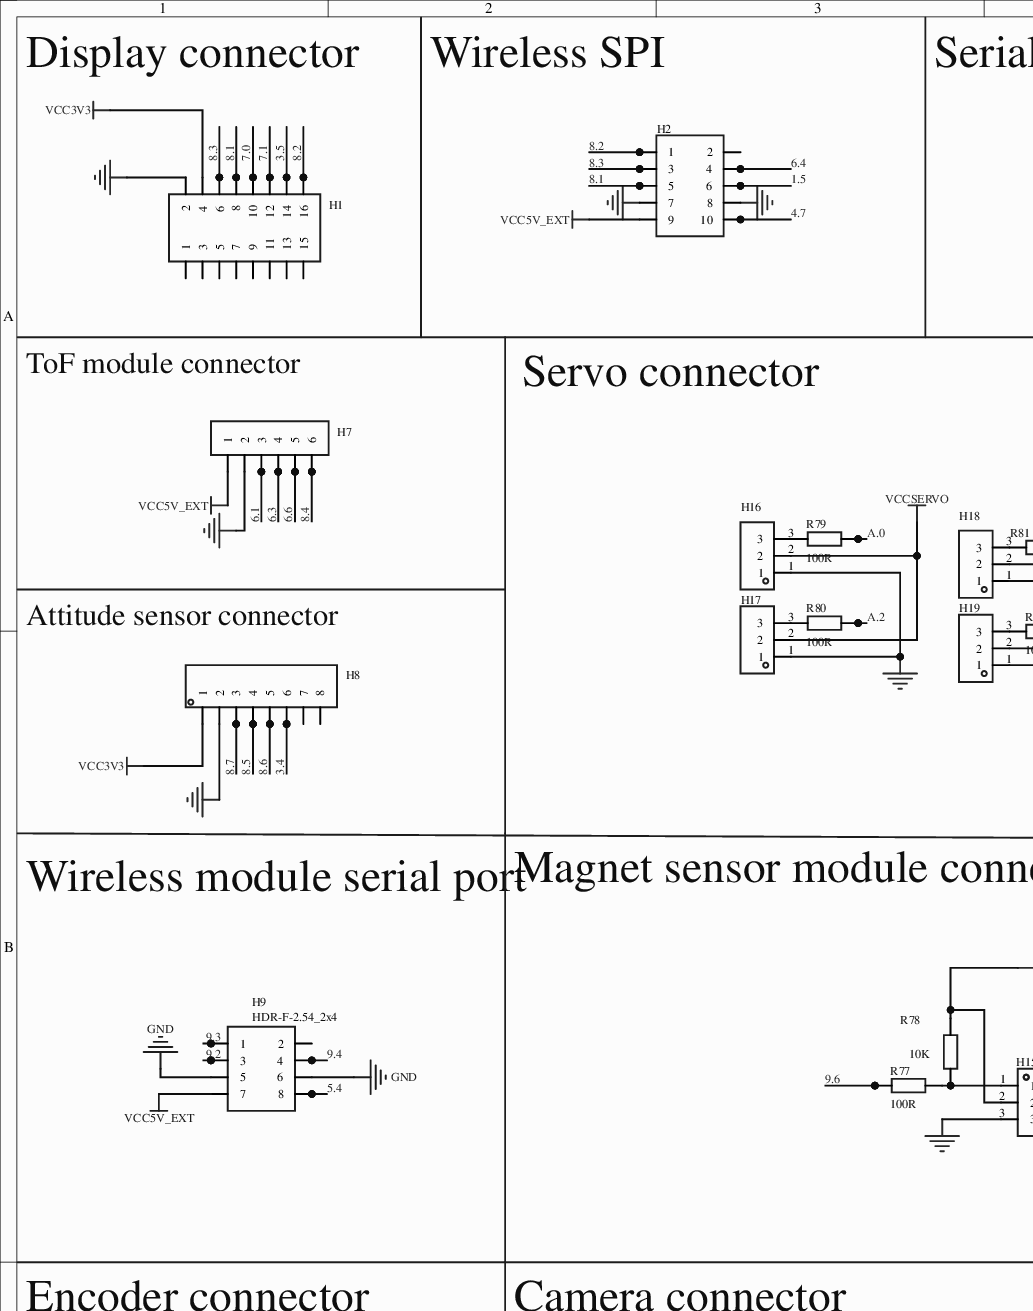
[diagram p0: MISC49918-4.schdoc, top left]
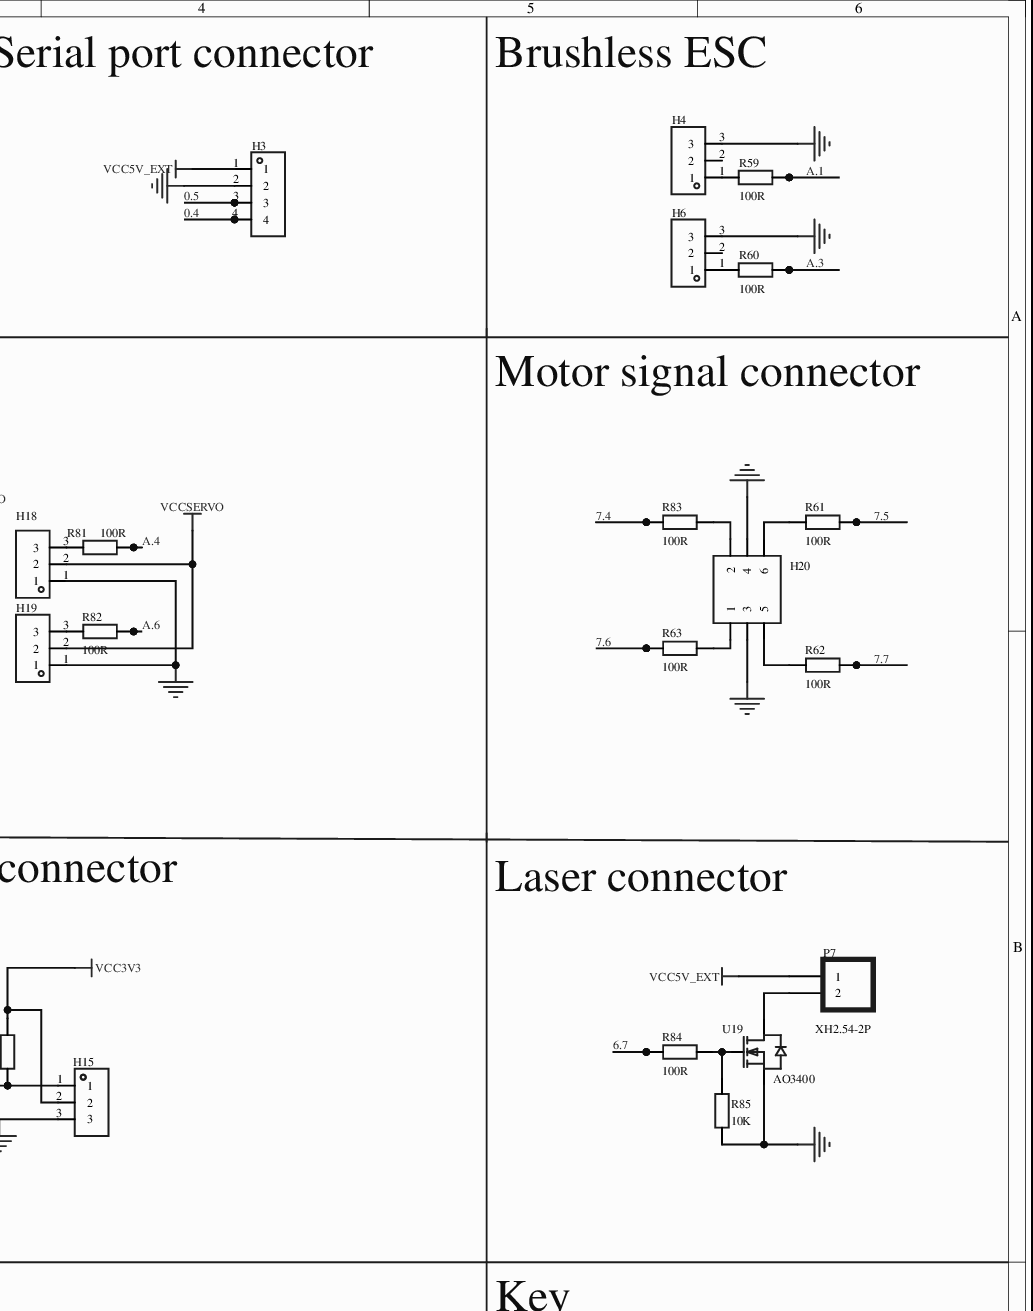
[diagram p1: MISC49918-4.schdoc, top right]
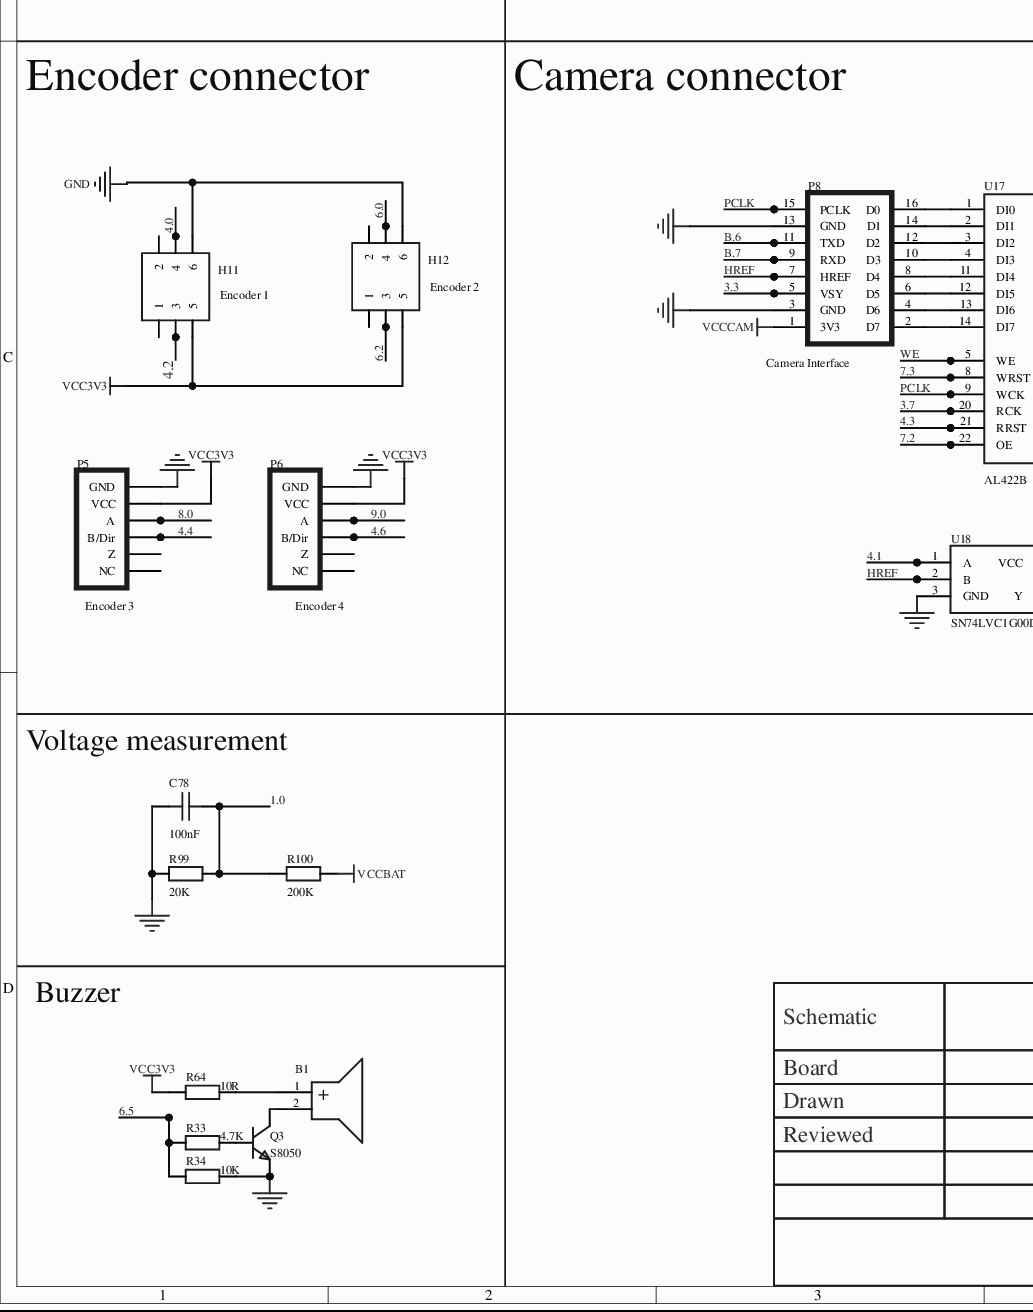
[diagram p2: MISC49918-4.schdoc, bottom left]
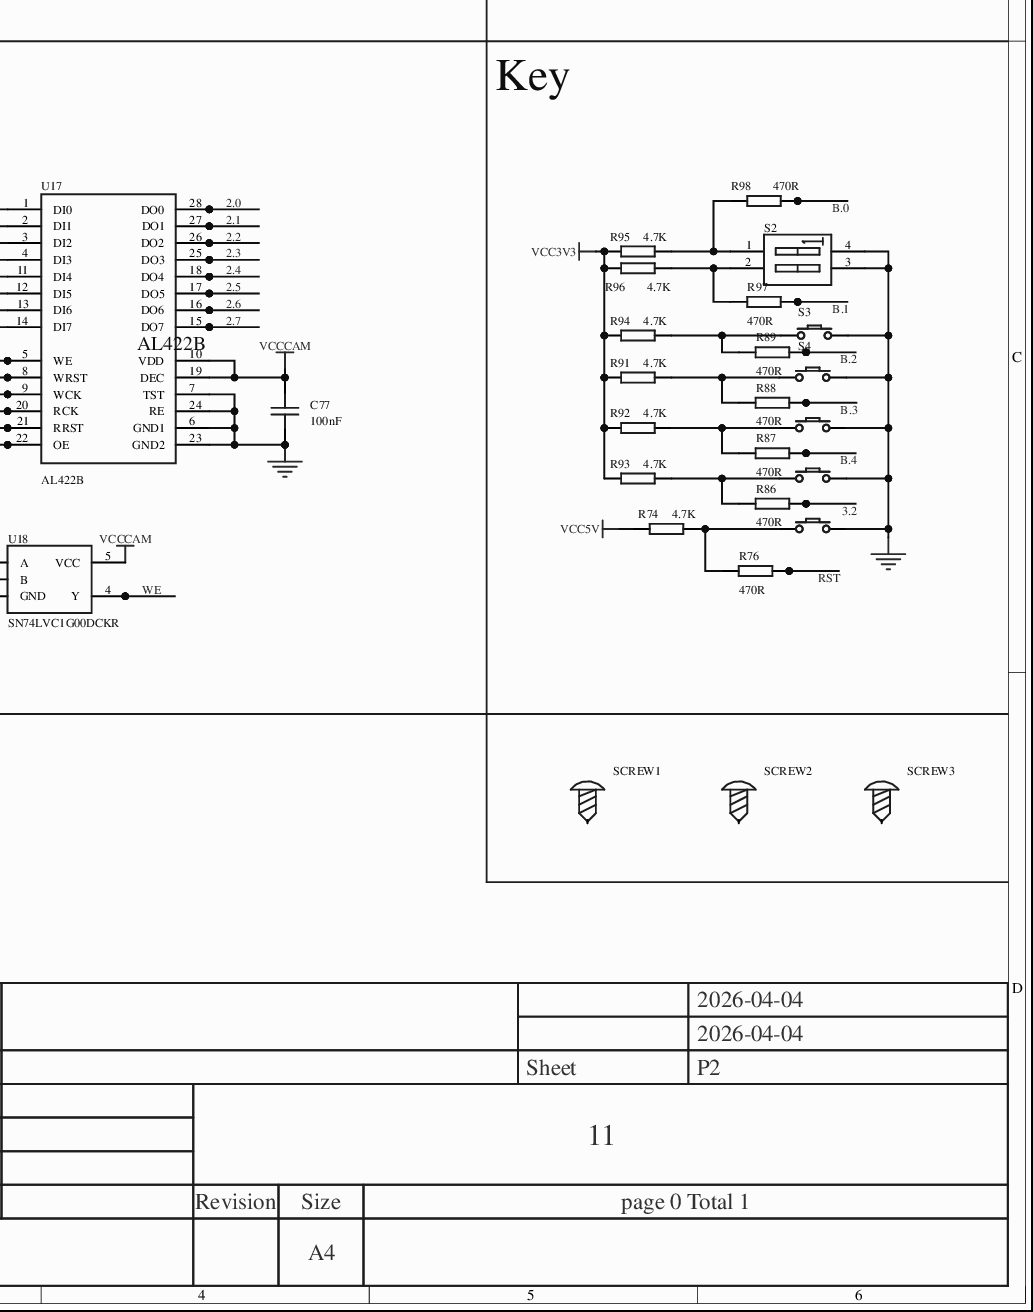
[diagram p3: MISC49918-4.schdoc, bottom right]
# Altium project MISC49918-2.PrjPcb (part 2 of 2)

## Sheet MISC49918-4.schdoc
size 297 x 381 mm; Version: V1.0; @Project Name: MISC49918; @Update Date: 2026-04-09; @Create Date: 2026-04-09; @Board Name: MISC49918; @Create Time: 13:05:40; @Page Count: 1; @Page No: 0; @Schematic Name: MISC49918; @Update Time: 13:05:40; Size: A4

### Parts
B1  3kHz  [BUZ-TH_BD9.0-P5.00-D0.6-FD]  (value not drawn)
C77  100nF  [C0603]
C78  100nF  [C0603]
H1  (no value)  [HDR-TH_16P-P2.54-V-F-R2-C8-S2.54-1]
H2  (no value)  [HDR-TH_10P-P2.54-V-F-R2-C5-S2.54]
H3  (no value)  [HDR-TH_4P-P2.54-V-M]
H4  (no value)  [HDR-TH_3P-P2.54-V-M]
H6  (no value)  [HDR-TH_3P-P2.54-V-M]
H7  (no value)  [HDR-TH_6P-P2.54-V-M-1]
H8  (no value)  [HDR-TH_8P-P2.54-V-M]
H9  HDR-F-2.54_2x4  [HDR-F-2.54_2X4]
H11  (no value)  [HDR-TH_6P-P2.54-V-R2-C3-S2.54_A2541WV-2X3P]
H12  (no value)  [HDR-TH_6P-P2.54-V-R2-C3-S2.54_A2541WV-2X3P]
H15  (no value)  [HDR-TH_3P-P2.54-V-M]
H16  (no value)  [HDR-TH_3P-P2.54-V-M]
H17  (no value)  [HDR-TH_3P-P2.54-V-M]
H18  (no value)  [HDR-TH_3P-P2.54-V-M]
H19  (no value)  [HDR-TH_3P-P2.54-V-M]
H20  (no value)  [HDR-TH_6P-P2.54-V-R2-C3-S2.54_A2541WV-2X3P]
P5  GH1.25-6P-SH new encoder board end, horizontal  [ECD-GH1.25-6P-SV]  (value not drawn)
P6  GH1.25-6P-SH new encoder board end, horizontal  [ECD-GH1.25-6P-SV]  (value not drawn)
P7  XH2.54-2P  [XH2.54-2P-DV]
P8  Camera Interface  [HDR2X8-F-High]
Q3  S8050  [SOT-23-3_L3.0-W1.7-P0.95-LS2.9-BR]
R33  4.7K  [R0603]
R34  10K  [R0603]
R59  100R  [R0603]
R60  100R  [R0603]
R61  100R  [R0603]
R62  100R  [R0603]
R63  100R  [R0603]
R64  10R  [R0603]
R74  4.7K  [RESC1608[0603]S-N]
R76  470R  [RESC1608[0603]S-N]
R77  100R  [R0603]
R78  10K  [R0603]
R79  100R  [R0603]
R80  100R  [R0603]
R81  100R  [R0603]
R82  100R  [R0603]
R83  100R  [R0603]
R84  100R  [R0603]
R85  10K  [R0603]
R86  470R  [RESC1608[0603]S-N]
R87  470R  [RESC1608[0603]S-N]
R88  470R  [RESC1608[0603]S-N]
R89  470R  [RESC1608[0603]S-N]
R91  4.7K  [RESC1608[0603]S-N]
R92  4.7K  [RESC1608[0603]S-N]
R93  4.7K  [RESC1608[0603]S-N]
R94  4.7K  [RESC1608[0603]S-N]
R95  4.7K  [RESC1608[0603]S-N]
R96  4.7K  [RESC1608[0603]S-N]
R97  470R  [RESC1608[0603]S-N]
R98  470R  [RESC1608[0603]S-N]
R99  20K  [R0603]
R100  200K  [R0603]
S2  SW DIP-2  [Code SW-2-DIP-2.54]  (value not drawn)
S3  KEY-TS1145  [TS-1199A]  (value not drawn)
S4  KEY-TS1145  [TS-1199A]  (value not drawn)
S5  KEY-TS1145  [TS-1199A]  (value not drawn)
S6  KEY-TS1145  [TS-1199A]  (value not drawn)
S7  KEY-TS1145  [TS-1199A]  (value not drawn)
SCREW1  (no value)  [M3螺丝]
SCREW2  (no value)  [M3螺丝]
SCREW3  (no value)  [M3螺丝]
U17  AL422B  [SOP-28]
U18  SN74LVC1G00DCKR  [SOT-353]
U19  AO3400  [SOT-23-3_L2.9-W1.3-P1.90-LS2.4-BL-2]

### Nets
GND: C77.1 C78.1 H1.2 H2.7 H2.8 H3.2 H4.3 H6.3 H7.2 H8.2 H9.5 H9.6 H11.6 H12.6 H15.3 H16.1 H17.1 H18.1 H19.1 H20.3 H20.4 P5.1(GND) P6.1(GND) P8.3(GND) P8.13(GND) Q3.2(E) R34.2 R85.1 R99.1 S2.3(B2) S2.4(B1) S3.1 S4.1 S5.1 S6.1 S7.1 U17.6(GND1) U17.7(TST) U17.23(GND2) U17.24(RE) U18.3(GND) U19.2(S)
VCC3V3: H1.4 H8.1 H11.5 H12.5 H15.2 P5.2(VCC) P6.2(VCC) R64.1 R78.2 R91.1 R92.1 R93.1 R94.1 R95.1 R96.1
VCC5V: R74.1
VCC5V_EXT: H2.9 H3.1 H7.1 H9.7 P7.1
VCCBAT: R100.2
VCCCAM: C77.2 P8.1(3V3) U17.10(VDD) U17.19(DEC) U18.5(VCC)
VCCSERVO: H16.2 H17.2 H18.2 H19.2
0.4: H3.4
0.5: H3.3
1.0: C78.2 R99.2 R100.1
1.5: H2.6
2.0: U17.28(DO0)
2.1: U17.27(DO1)
2.2: U17.26(DO2)
2.3: U17.25(DO3)
2.4: U17.18(DO4)
2.5: U17.17(DO5)
2.6: U17.16(DO6)
2.7: U17.15(DO7)
3.2: R86.1
3.3: P8.5(VSY)
3.4: H8.6
3.5: H1.14
3.7: U17.20(RCK)
4.0: H11.4
4.1: U18.1(A)
4.2: H11.3
4.3: U17.21(RRST)
4.4: P5.4(B/Dir)
4.6: P6.4(B/Dir)
4.7: H2.10
5.4: H9.8
6.0: H12.4
6.1: H7.3
6.2: H12.3
6.3: H7.4
6.4: H2.4
6.5: R33.1 R34.1
6.6: H7.5
6.7: R84.1
7.0: H1.10
7.1: H1.12
7.2: U17.22(OE)
7.3: U17.8(WRST)
7.4: R83.1
7.5: R61.2
7.6: R63.1
7.7: R62.2
8.0: P5.3(A)
8.1: H1.8 H2.5
8.2: H1.16 H2.1
8.3: H1.6 H2.3
8.4: H7.6
8.5: H8.4
8.6: H8.5
8.7: H8.3
9.0: P6.3(A)
9.2: H9.3
9.3: H9.1
9.4: H9.4
9.6: R77.1
A.0: R79.2
A.1: R59.2
A.2: R80.2
A.3: R60.2
A.4: R81.2
A.6: R82.2
B.0: R98.1
B.1: R97.1
B.2: R89.1
B.3: R88.1
B.4: R87.1
B.6: P8.11(TXD)
B.7: P8.9(RXD)
HREF: P8.7(HREF) U18.2(B)
PCLK: P8.15(PCLK) U17.9(WCK)
RST: R76.1
WE: U17.5(WE) U18.4(Y)
NetB1_1: B1.1(+) R64.2
NetB1_2: B1.2(-) Q3.3(C)
NetH4_1: H4.1 R59.1
NetH6_1: H6.1 R60.1
NetH15_1: H15.1 R77.2 R78.1
NetH16_3: H16.3 R79.1
NetH17_3: H17.3 R80.1
NetH18_3: H18.3 R81.1
NetH19_3: H19.3 R82.1
NetH20_1: H20.1 R63.2
NetH20_2: H20.2 R83.2
NetH20_5: H20.5 R62.1
NetH20_6: H20.6 R61.1
NetP7_2: P7.2 U19.3(D)
NetP8_2: P8.2(D7) U17.14(DI7)
NetP8_4: P8.4(D6) U17.13(DI6)
NetP8_6: P8.6(D5) U17.12(DI5)
NetP8_8: P8.8(D4) U17.11(DI4)
NetP8_10: P8.10(D3) U17.4(DI3)
NetP8_12: P8.12(D2) U17.3(DI2)
NetP8_14: P8.14(D1) U17.2(DI1)
NetP8_16: P8.16(D0) U17.1(DI0)
NetQ3_1: Q3.1(B) R33.2
NetR74_2: R74.2 R76.2 S7.2
NetR84_2: R84.2 R85.2 U19.1(G)
NetR86_2: R86.2 R93.2 S6.2
NetR87_2: R87.2 R92.2 S5.2
NetR88_2: R88.2 R91.2 S4.2
NetR89_2: R89.2 R94.2 S3.2
NetR95_2: R95.2 R98.2 S2.1(A1)
NetR96_2: R96.2 R97.2 S2.2(A2)

Not connected (* = marked no-connect by the designer): H1 1* 3* 5* 7* 9* 11* 13* 15*; H2 2*; H4 2*; H6 2*; H8 7* 8*; H9 2*; H11 1* 2*; H12 1* 2*; P5 5(Z)* 6(NC)*; P6 5(Z)* 6(NC)*; SCREW1 1*; SCREW2 1*; SCREW3 1*

### Notes on the sheet
- Display connector
- Wireless SPI
- Serial port connector
- Brushless ESC
- ToF module connector
- Servo connector
- Motor signal connector
- Attitude sensor connector
- Wireless module serial port
- Magnet sensor module connector
- Laser connector
- Encoder connector
- Camera connector
- Key
- (near H11) Encoder 1
- (near H12) Encoder 2
- (near P5) Encoder 3
- (near P6) Encoder 4
- (near C78) Voltage measurement
- Buzzer
- 2026-04-04
- Schematic
- Board
- Sheet
- P2
- Drawn
- Reviewed
- 11
- Revision
- Size
- A4
- page 0 Total 1

### Library data of the parts
B1 = HNB09A03: Drive method: active (built-in driver circuit); Construction: electromagnetic; Frequency: 3kHz; Sound pressure (SPL): 85dB@10cm;; Manufacturer: 华能; 3D Model: 13273335caac486e928bafb4d9fdf12d; 3D Model Transform: 354.33,354.33,0,90,0,0,-0.005,0,-177.165; Operating Voltage: 1.5V~4.5V; Current Consumption: 30mA; AddInBom: yes; ModelName: BUZ-TH_D9.0-H5.5-P5.0; Device: HNB09A03; Symbol: HNB09A03; LCSC Part Name: 电磁式有源一体蜂鸣器HNB09A03; Supplier Footprint: 插件,D=9mm; Datasheet: https://atta.szlcsc.com/upload/public/pdf/source/20170522/1495448326172.pdf; Oscillator Circuit: Active (built-in driver circuit); Technology Type: Electromagnetic; Sound Pressure Level (SPL): 85dB@10cm; Diameter (φD): 9mm; Length: -; Width: -; Height: 5.5mm; Operating Temperature: -20℃~+70℃; Supplier: LCSC; Supplier Part: C96102; Manufacturer Part: HNB09A03; Value: 3kHz; FootprintName: BUZ-TH_BD9.0-P5.00-D0.6-FD; ConvertToPcb: yes
C77 C78 = CAP_0603: Symbol: Capacitance; 3D Model: ac125912035d415993ca9572d50418b1; 3D Model Transform: 62.992,31.496,0,0,0,0,0,0,0; ConvertToPcb: yes; ModelName: C0603_L1.6-W0.8-H0.8; Device: CAP_0603; Supplier Footprint: 0603; Value: 100nF; FootprintName: C0603; AddInBom: yes
H1 = HDR-F_2.54_2x8: Symbol: HDR-F-2.54_2x8; 3D Model: f6b5f7d40ec74b809fbaeebc5002f6e0; 3D Model Transform: 799.99844,200,0,0,0,0,0,0,-118.11; ConvertToPcb: yes; ModelName: HDR2.54-F-LI-2X8P; Device: HDR-F_2.54_2x8; Supplier Part: C30734; Supplier Footprint: 插件; FootprintName: HDR-TH_16P-P2.54-V-F-R2-C8-S2.54-1; AddInBom: yes
H2 = HDR-F_2.54_2x5: Symbol: HDR-F-2.54_2x5; 3D Model: 86e5d65f54dd476391caab3fdb916824; 3D Model Transform: 499.999,200,0,0,0,0,0,0,-118.11; ConvertToPcb: yes; ModelName: HDR2.54-F-LI-2X5P; Device: HDR-F_2.54_2x5; Supplier Part: C92270; Supplier Footprint: 插件; FootprintName: HDR-TH_10P-P2.54-V-F-R2-C5-S2.54; AddInBom: yes
H3 = HDR-M_2.54_1x4P: Symbol: PZ254V-11-04P; 3D Model: 112f4d05e8d64e99ab9a333894bea4f9; 3D Model Transform: 399.999,104.7242,0,0,0,0,0,0,-118.11; ConvertToPcb: yes; ModelName: HDR-TH_4P-P2.54-M-LI-1X4P; Device: HDR-M_2.54_1x4P; Supplier Part: C492403; Supplier Footprint: 插件; FootprintName: HDR-TH_4P-P2.54-V-M; AddInBom: yes
H4 H6 H15-H19 = HDR-M_2.54_1x3P: 3D Model: bb473b6d38ff42a99216a4fcdbdcc4cb; 3D Model Transform: 299.9993964861481,99.99979882871602,454.3297999999999,0,0,0,0,0,-118.11024; AddInBom: yes; ModelName: HDR-TH_3P-P2.54-M-LI-1X3P; Device: HDR-M_2.54_1x3P; Symbol: HDR-M_2.54_1x3P; Supplier Part: C2937625; Supplier Footprint: 插件; FootprintName: HDR-TH_3P-P2.54-V-M; ConvertToPcb: yes
H7 = HDR-M_2.54_1x6P: Symbol: Header-Male-2.54_1x6; 3D Model: 60739dffc9b04830a286435b0fefbd4a; 3D Model Transform: 599.999,100,0,0,0,0,0,0,-118.11; ConvertToPcb: yes; ModelName: HDR2.54-M-LI-1X6P; Device: HDR-M_2.54_1x6P; Supplier Part: C37208; Supplier Footprint: 插件; FootprintName: HDR-TH_6P-P2.54-V-M-1; AddInBom: yes
H8 = HDR-M_2.54_1x8P: Symbol: Header-Male-2.54_1x8; 3D Model: f5b96e27511e49e38545e53df2320202; 3D Model Transform: 807.87244,98.425,0,0,0,0,0,0,-118.11; ConvertToPcb: yes; Device: HDR-M_2.54_1x8P; Supplier Part: C124381; Supplier Footprint: 插件; FootprintName: HDR-TH_8P-P2.54-V-M; AddInBom: yes; ModelName: HDR-TH_8P-P2.54-V-M
H9 = HDR-F-2.54_2x4: Add into BOM: yes; Contributor: LCEDA_Lib; ModelId: ff59f67622f24105899cab48d077d597; ModelTransform: 0,0,0,0,0,0,0,0,0; Device: HDR-F-2.54_2x4; Symbol: HDR-F-2.54_2x4; Convert to PCB: yes; Origin Footprint: HDR-F-2.54_2X4; Supplier Part: C239344; Supplier: LCSC; spicePre: H; spiceSymbolName: HDR-F-2.54_2x4; FootprintName: HDR-F-2.54_2X4; ModelName: HDR-F-2.54_2x4
H11 H12 H20 = HDR-M_2.54_2x3: Symbol: HDR-M-2.54_2x3; 3D Model: fd1b55b786fb415ca65c4187088147b7; 3D Model Transform: 299.9994,200,0,0,0,0,0,0,-118.11; ConvertToPcb: yes; ModelName: HDR2.54-M-LI-2x3P; Device: HDR-M_2.54_2x3; Supplier Part: C402781; Supplier Footprint: 插件,P=2.54mm; FootprintName: HDR-TH_6P-P2.54-V-R2-C3-S2.54_A2541WV-2X3P; AddInBom: yes
P5 P6 = GH1.25-6P-SH新编码器主板端-卧式: Seekfree 1024-line encoder GH1.25-6P mainboard end, horizontal; componentDisplayMode: -1; AddInBom: yes; Device: GH1.25-6P-SH new encoder board end, horizontal; Symbol: GH1.25-6P-SH new encoder board end, horizontal; Revision: V1.0; Value: GH1.25-6P; Footprint Name: ECD-GH1.25-6P-SV; ConvertToPcb: yes
P7 = XH2.54-2P: componentDisplayMode: -1; AddInBom: yes; Device: XH2.54-2P; Symbol: XH2.54-2P; Revision: V1.0; Value: XH2.54-2P; Footprint Name: XH2.54-2P-SV; ConvertToPcb: yes; Description: XH2.54-2P
P8 = Camera Interface: Camera adapter board connector 2x8 dual-row socket; componentDisplayMode: -1; AddInBom: yes; Device: Camera Interface; Symbol: Camera Interface; LatestRevisionDate: 17-Jul-2002; LatestRevisionNote: Re-released for DXP Platform.; Price(RMB): 0.00; Footprint Name: Cam_HDR2X8-F-SMT; ConvertToPcb: yes; Publisher: Altium Limited
Q3 = S8050 J3Y_C2146: Transistor type: NPN; Collector current (Ic): 500mA; Collector-emitter breakdown voltage (Vceo): 25V; Power (Pd): 300mW; DC current gain (hFE@Ic,Vce): 200@50mA,1V;; Manufacturer: CJ(江苏长电/长晶); Symbol: S8050_C2146; 3D Model: 89cb27a44ab2466697082bb9fd73a7d0; 3D Model Transform: 114.173,110.236,0,90,0,0,0,0,0; Transition Frequency (fT): 150MHz; Collector Cut-Off Current (Icbo): 100nA; Collector-Emitter Saturation Voltage (VCE(sat)@Ic,Ib): 600mV@500mA,50mA; AddInBom: yes; ModelName: SOT-23-3L_L2.9-W1.6-H1.1-LS2.8-P0.95; Device: S8050 J3Y_C2146; Manufacturer Part: S8050; LCSC Part Name: S8050 J3Y(RANGE:200-350) H档(200-350); Supplier Part: C2146; Supplier Footprint: SOT-23; Datasheet: https://atta.szlcsc.com/upload/public/pdf/source/20140809/1457707209234.pdf; Supplier: LCSC; Transistor Type: NPN; Collector Current (Ic): 500mA; Collector-Emitter Breakdown Voltage (Vceo): 25V; Power Dissipation (Pd): 300mW; DC Current Gain (hFE@Ic,Vce): 200@50mA,1V; Operating Temperature: -; FootprintName: SOT-23-3_L3.0-W1.7-P0.95-LS2.9-BR; ConvertToPcb: yes
R33 R34 R59-R64 R77-R85 R99 R100 = Res_0603: Symbol: Resistor; 3D Model: fc143cca1e79419f9cd78b61e9279f08; 3D Model Transform: 31.8897,63.7794,0,90,0,0,0,0,0; ConvertToPcb: yes; Device: Res_0603; Supplier Footprint: 0603; FootprintName: R0603; AddInBom: yes; ModelName: R0603
  R33: Value: 4.7K
  R34 R78 R85: Value: 10K
  R59-R63 R77 R79-R84: Value: 100R
  R64: Value: 10R
  R99: Value: 20K
  R100: Value: 200K
R74 R76 R86-R89 R91-R98 = Res-Chip_5: Tolerance: ±1%; Origin Footprint 2: RESC0603[0201]-L; Origin Footprint 3: RESC0603[0201]-M; Origin Footprint 4: RESC0603[0201]-N; Origin Footprint 5: RESC0603[0201]S-L; Origin Footprint 6: RESC0603[0201]S-M; Origin Footprint 7: RESC0603[0201]S-N; Origin Footprint 8: RESC1005[0402]-L; Origin Footprint 9: RESC1005[0402]-M; Origin Footprint 10: RESC1005[0402]-N; Origin Footprint 11: RESC1005[0402]S-L; Origin Footprint 12: RESC1005[0402]S-M; Origin Footprint 13: RESC1005[0402]S-N; Origin Footprint 14: RESC1608[0603]-L; Origin Footprint 15: RESC1608[0603]-M; Origin Footprint 16: RESC1608[0603]-N; Origin Footprint 17: RESC1608[0603]S-L; Origin Footprint 18: RESC1608[0603]S-M; Origin Footprint 19: RESC2012[0805]; Origin Footprint 20: RESC2012[0805]S-L; Origin Footprint 21: RESC2012[0805]S-M; Origin Footprint 22: RESC2012[0805]S-N; Origin Footprint 23: RESC3216[1206]; Origin Footprint 24: RESC3216[1206]S-L; Origin Footprint 25: RESC3216[1206]S-M; Origin Footprint 26: RESC3216[1206]S-N; Origin Footprint 27: RESC3225[1210]; Origin Footprint 28: RESC3225[1210]S; Origin Footprint 29: RESC5025[2010]; Origin Footprint 30: RESC5025[2010]S; Origin Footprint 31: RESC6332[2512]; Origin Footprint 32: RESC6332[2512]S; Origin Footprint 33: RESC0402[01005]-L; AddInBom: yes; Device: Res-Chip_5; Symbol: Res-Chip_5; Revision: V1.0; FootprintName: RESC1608[0603]S-N; ConvertToPcb: yes
  R74 R91-R96: Value: 4.7K
  R76 R86-R89 R97 R98: Value: 470R
S2 = Code SW-2: Origin Footprint 2: Code SW-2-SMD-1.27; AddInBom: yes; Device: Code SW-2; Symbol: Code SW-2; Published: 24-Mar-1999; Revision: July-2002: Re-released for DXP Platform.; Price(RMB): 0.000; FootprintName: Code SW-2-DIP-2.54; ConvertToPcb: yes; Publisher: Altium Limited
S3-S7 = KEY-TS1145: Origin Footprint 2: TS1145-C-A; AddInBom: yes; Device: KEY-TS1145; Symbol: KEY-TS1145; Revision: V1.0; Value: KEY-TS1145; FootprintName: TS-1199A; ConvertToPcb: yes
SCREW1-SCREW3 = M3螺丝: Device: M3 screw; Symbol: Screw hole; ConvertToPcb: yes; Supplier Footprint: 插件; FootprintName: M3 screw; AddInBom: yes
U17 = AL422B: 8-channel FIFO memory; componentDisplayMode: -1; AddInBom: yes; Device: AL422B; Symbol: AL422B; Revision: V1.0; Value: AL422B; Footprint Name: SOP-28; ConvertToPcb: yes
U18 = SN74LVC1G00DCKR: SN74LVC1G00DCKR NAND gate; componentDisplayMode: -1; AddInBom: yes; Device: SN74LVC1G00DCKR; Symbol: SN74LVC1G00DCKR; Footprint Name: SOT-353; ConvertToPcb: yes
U19 = AO3400: Symbol: AO3400_C9900013365; 3D Model: 115ef394a879442d90491e6127930138; 3D Model Transform: 114.173,94.488,0,0,0,0,0,0,0; AddInBom: yes; ModelName: SOT-23-3_L2.9-W1.3-P1.90-LS2.4; Device: AO3400; LCSC Part Name: AO3400; Supplier Part: C9900013365; Manufacturer Part: AO3400; Supplier Footprint: SOT-23; JLCPCB Part Class: Extended library; Supplier: LCSC; FootprintName: SOT-23-3_L2.9-W1.3-P1.90-LS2.4-BL-2; ConvertToPcb: yes

## Nets that join several sheets
GND: MISC49918-3 (44 pins), MISC49918-4 (42 pins)
VCC3V3: MISC49918-3 (C74.2 C76.2 R58.1 U16.5), MISC49918-4 (15 pins)
VCC5V: MISC49918-3 (11 pins), MISC49918-4 (R74.1)
VCC5V_EXT: MISC49918-3 (C29.2 R21.1 U7.1), MISC49918-4 (5 pins)
VCCBAT: MISC49918-3 (8 pins), MISC49918-4 (R100.2)
VCCCAM: MISC49918-3 (C43.2 C72.2 R18.1 U4.5), MISC49918-4 (5 pins)
VCCSERVO: MISC49918-3 (6 pins), MISC49918-4 (H16.2 H17.2 H18.2 H19.2)
0.4: MISC49918-3 (U1.63), MISC49918-4 (H3.4)
0.5: MISC49918-3 (U1.68), MISC49918-4 (H3.3)
1.0: MISC49918-3 (U1.82), MISC49918-4 (C78.2 R99.2 R100.1)
1.5: MISC49918-3 (U1.85), MISC49918-4 (H2.6)
2.0: MISC49918-3 (U1.37), MISC49918-4 (U17.28)
2.1: MISC49918-3 (U1.40), MISC49918-4 (U17.27)
2.2: MISC49918-3 (U1.39), MISC49918-4 (U17.26)
2.3: MISC49918-3 (U1.42), MISC49918-4 (U17.25)
2.4: MISC49918-3 (U1.41), MISC49918-4 (U17.18)
2.5: MISC49918-3 (U1.44), MISC49918-4 (U17.17)
2.6: MISC49918-3 (U1.43), MISC49918-4 (U17.16)
2.7: MISC49918-3 (U1.46), MISC49918-4 (U17.15)
3.2: MISC49918-3 (U1.13), MISC49918-4 (R86.1)
3.3: MISC49918-3 (U1.16), MISC49918-4 (P8.5)
3.4: MISC49918-3 (U1.15), MISC49918-4 (H8.6)
3.5: MISC49918-3 (U1.20), MISC49918-4 (H1.14)
3.7: MISC49918-3 (U1.21), MISC49918-4 (U17.20)
4.0: MISC49918-3 (U1.89), MISC49918-4 (H11.4)
4.1: MISC49918-3 (U1.35), MISC49918-4 (U18.1)
4.2: MISC49918-3 (U1.34), MISC49918-4 (H11.3)
4.3: MISC49918-3 (U1.36), MISC49918-4 (U17.21)
4.4: MISC49918-3 (U1.38), MISC49918-4 (P5.4)
4.6: MISC49918-3 (U1.60), MISC49918-4 (P6.4)
4.7: MISC49918-3 (U1.84), MISC49918-4 (H2.10)
5.4: MISC49918-3 (U1.90), MISC49918-4 (H9.8)
6.0: MISC49918-3 (U1.69), MISC49918-4 (H12.4)
6.1: MISC49918-3 (U1.71), MISC49918-4 (H7.3)
6.2: MISC49918-3 (U1.72), MISC49918-4 (H12.3)
6.3: MISC49918-3 (U1.73), MISC49918-4 (H7.4)
6.4: MISC49918-3 (U1.92), MISC49918-4 (H2.4)
6.5: MISC49918-3 (U1.91), MISC49918-4 (R33.1 R34.1)
6.6: MISC49918-3 (U1.94), MISC49918-4 (H7.5)
6.7: MISC49918-3 (U1.93), MISC49918-4 (R84.1)
7.0: MISC49918-3 (U1.22), MISC49918-4 (H1.10)
7.1: MISC49918-3 (U1.23), MISC49918-4 (H1.12)
7.2: MISC49918-3 (U1.24), MISC49918-4 (U17.22)
7.3: MISC49918-3 (U1.25), MISC49918-4 (U17.8)
7.4: MISC49918-3 (U1.45), MISC49918-4 (R83.1)
7.5: MISC49918-3 (U1.47), MISC49918-4 (R61.2)
7.6: MISC49918-3 (U1.48), MISC49918-4 (R63.1)
7.7: MISC49918-3 (U1.49), MISC49918-4 (R62.2)
8.0: MISC49918-3 (U1.74), MISC49918-4 (P5.3)
8.1: MISC49918-3 (U1.75), MISC49918-4 (H1.8 H2.5)
8.2: MISC49918-3 (U1.76), MISC49918-4 (H1.16 H2.1)
8.3: MISC49918-3 (U1.77), MISC49918-4 (H1.6 H2.3)
8.4: MISC49918-3 (U1.78), MISC49918-4 (H7.6)
8.5: MISC49918-3 (U1.79), MISC49918-4 (H8.4)
8.6: MISC49918-3 (U1.80), MISC49918-4 (H8.5)
8.7: MISC49918-3 (U1.81), MISC49918-4 (H8.3)
9.0: MISC49918-3 (U1.6), MISC49918-4 (P6.3)
9.2: MISC49918-3 (U1.8), MISC49918-4 (H9.3)
9.3: MISC49918-3 (U1.9), MISC49918-4 (H9.1)
9.4: MISC49918-3 (U1.10), MISC49918-4 (H9.4)
9.6: MISC49918-3 (U1.11), MISC49918-4 (R77.1)
A.0: MISC49918-3 (U1.26), MISC49918-4 (R79.2)
A.1: MISC49918-3 (U1.27), MISC49918-4 (R59.2)
A.2: MISC49918-3 (U1.28), MISC49918-4 (R80.2)
A.3: MISC49918-3 (U1.29), MISC49918-4 (R60.2)
A.4: MISC49918-3 (U1.30), MISC49918-4 (R81.2)
A.6: MISC49918-3 (U1.32), MISC49918-4 (R82.2)
B.0: MISC49918-3 (U1.50), MISC49918-4 (R98.1)
B.1: MISC49918-3 (U1.51), MISC49918-4 (R97.1)
B.2: MISC49918-3 (U1.52), MISC49918-4 (R89.1)
B.3: MISC49918-3 (U1.53), MISC49918-4 (R88.1)
B.4: MISC49918-3 (U1.54), MISC49918-4 (R87.1)
B.6: MISC49918-3 (U1.56), MISC49918-4 (P8.11)
B.7: MISC49918-3 (U1.57), MISC49918-4 (P8.9)
RST: MISC49918-3 (U1.5 U4.3 U7.4 U16.3), MISC49918-4 (R76.1)